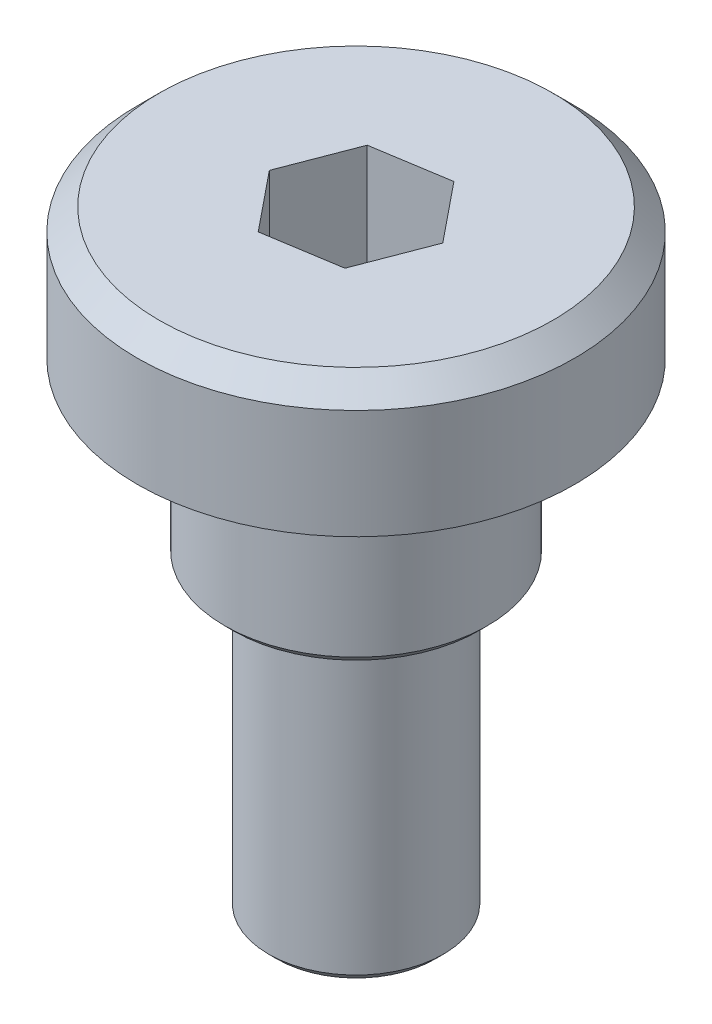
SolidWorks part; units mm, degrees
ref_plane "Front" through (0, 0, 0) normal (0, 0, 1) x (1, 0, 0)
ref_plane "Top" through (0, 0, 0) normal (0, 1, 0) x (1, 0, 0)
ref_plane "Right" through (0, 0, 0) normal (1, 0, 0) x (0, 0, -1)
sketch "草图1" plane through (0, 0, 0) normal (0, 1, 0) x (1, 0, 0)
  circle A0 centre (0, 0) radius 2
  dimension "D1" = 4
extrude "凸台-拉伸1" add sketch "草图1" along normal blind 7
cosmetic thread "装饰螺纹线1" parameters "D1"=7, "D2"=3.242
sketch "草图2" plane through (0, 7, 0) normal (0, 1, 0) x (1, 0, 0)
  circle A0 centre (0, 0) radius 3
  dimension "D1" = 6
extrude "凸台-拉伸2" add sketch "草图2" along normal blind 4
sketch "草图3" plane through (0, 11, 0) normal (0, 1, 0) x (1, 0, 0)
  circle A0 centre (0, 0) radius 5
  dimension "D1" = 10
extrude "凸台-拉伸3" add sketch "草图3" along normal blind 3
chamfer "倒角1" distance 0.5 angle 45 1 edges at (0, 14, 5)
chamfer "倒角2" distance 0.2 angle 45 1 edges at (0, 7, 3)
chamfer "倒角3" distance 0.2 angle 45 1 edges at (0, 0, 2)
sketch "草图4" plane through (0, 14, 0) normal (0, 1, 0) x (1, 0, 0)
  line L1 (1.0908, -1.3454) -> (1.7106, 0.272)
  line L2 (1.7106, 0.272) -> (0.6197, 1.6174)
  line L3 (0.6197, 1.6174) -> (-1.0908, 1.3454)
  line L4 (-1.0908, 1.3454) -> (-1.7106, -0.272)
  line L5 (-1.7106, -0.272) -> (-0.6197, -1.6174)
  line L6 (-0.6197, -1.6174) -> (1.0908, -1.3454)
  circle A0 centre (0, 0) radius 1.5 construction
  dimension "D1" = 3
extrude "切除-拉伸1" cut sketch "草图4" against normal blind 3
